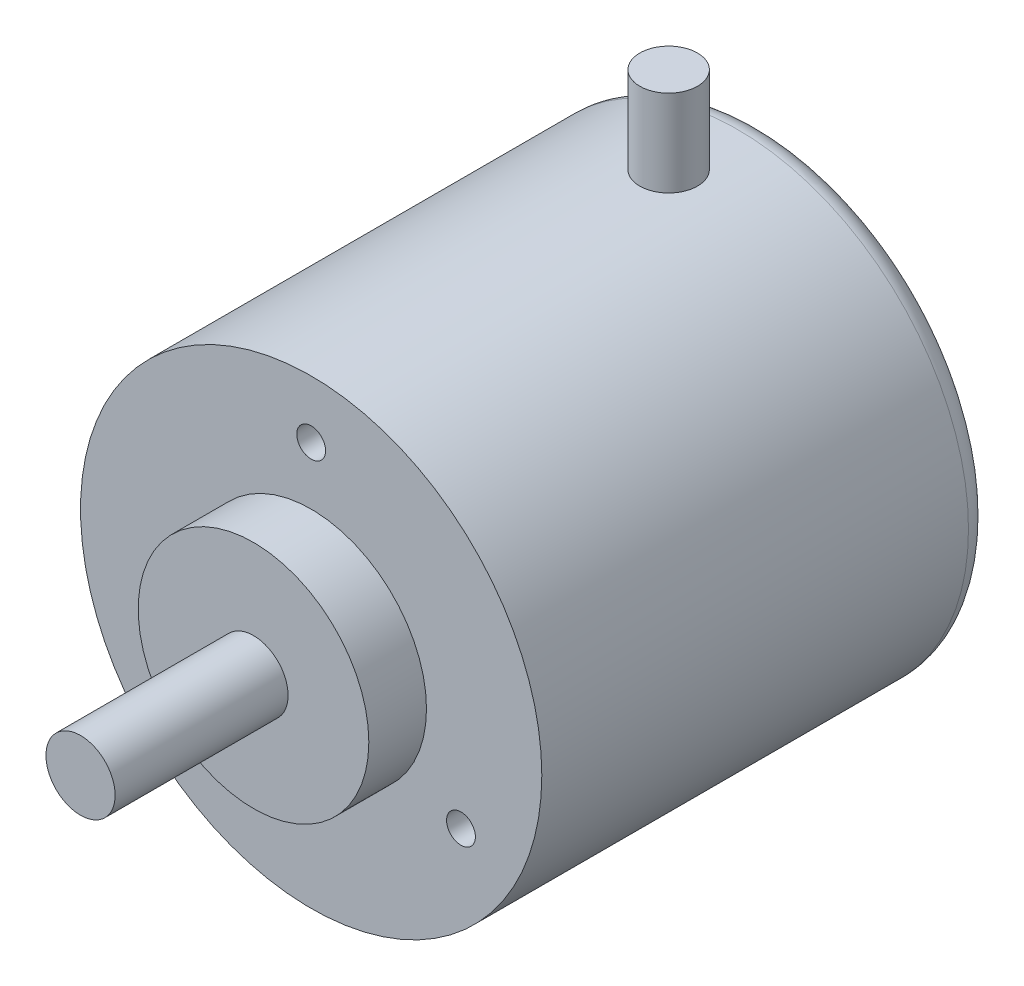
from build123d import *

# Parameters (mm, degrees)
SKETCH_1_R                  = 20
EXTRUDE_1_DEPTH             = 39
SKETCH_2_R                  = 10
EXTRUDE_2_DEPTH             = 5
SKETCH_3_R                  = 3
EXTRUDE_3_DEPTH             = 15
HOLE_WIZARD_M3_1_AT_2_COUNT = 2
HOLE_WIZARD_M3_1_AT_2_PITCH = 25.980762114
HOLE_WIZARD_M3_1_AT_3_COUNT = 2
HOLE_WIZARD_M3_1_AT_3_PITCH = 25.980762114
FILLET_1_R                  = 2
SKETCH_8_R                  = 2.5
EXTRUDE_4_DEPTH             = 7.5


with BuildPart() as part:
    # 草图1 → 凸台-拉伸1 (new body)
    with BuildSketch(Plane.XY):
        Circle(SKETCH_1_R)
    extrude(amount=EXTRUDE_1_DEPTH)

    # 草图6 → M3 螺纹孔1 (revolve, cut)
    with BuildSketch(Plane(origin=(0, 15, 39), x_dir=(0, -1, 0), z_dir=(1, 0, 0))):
        Polygon((0, 0), (0, 7.5), (1.25, 6.748924226), (1.25, 0), align=None)
    hole_wizard_m3_1 = revolve(axis=Axis((0, 15, 45.35), (0, 0, -1)), mode=Mode.SUBTRACT)

    # M3 螺纹孔1 at 2: M3 螺纹孔1 ×2
    with Locations(*[Vector(-0.49999999999996314, -0.8660254037844599, 0) * (i * HOLE_WIZARD_M3_1_AT_2_PITCH) for i in range(1, HOLE_WIZARD_M3_1_AT_2_COUNT)]):
        add(hole_wizard_m3_1, mode=Mode.SUBTRACT)

    # M3 螺纹孔1 at 3: M3 螺纹孔1 ×2
    with Locations(*[Vector(0.5000000000000372, -0.8660254037844173, 0) * (i * HOLE_WIZARD_M3_1_AT_3_PITCH) for i in range(1, HOLE_WIZARD_M3_1_AT_3_COUNT)]):
        add(hole_wizard_m3_1, mode=Mode.SUBTRACT)

    # 圆角1
    fillet_1_edges = [part.edges().sort_by_distance(p)[0] for p in [
        (-20, 0, 0),
    ]]
    fillet(fillet_1_edges, radius=FILLET_1_R)


with BuildPart() as body_2:
    # 草图2 → 凸台-拉伸2 (new body)
    with BuildSketch(Plane.XY.offset(39)):
        Circle(SKETCH_2_R)
    extrude(amount=EXTRUDE_2_DEPTH)


with BuildPart() as body_3:
    # 草图3 → 凸台-拉伸3 (new body)
    with BuildSketch(Plane.XY.offset(44)):
        Circle(SKETCH_3_R)
    extrude(amount=EXTRUDE_3_DEPTH)


with BuildPart() as body_4:
    # 草图8 → 凸台-拉伸4 (new body)
    with BuildSketch(Plane(origin=(0, 20, 0), x_dir=(1, 0, 0), z_dir=(0, 1, 0))):
        with Locations(Location((0, -8, 0), (0, 0, 270))):
            Circle(SKETCH_8_R)
    extrude(amount=EXTRUDE_4_DEPTH)


solid = Compound([part.part, body_2.part, body_3.part, body_4.part])
